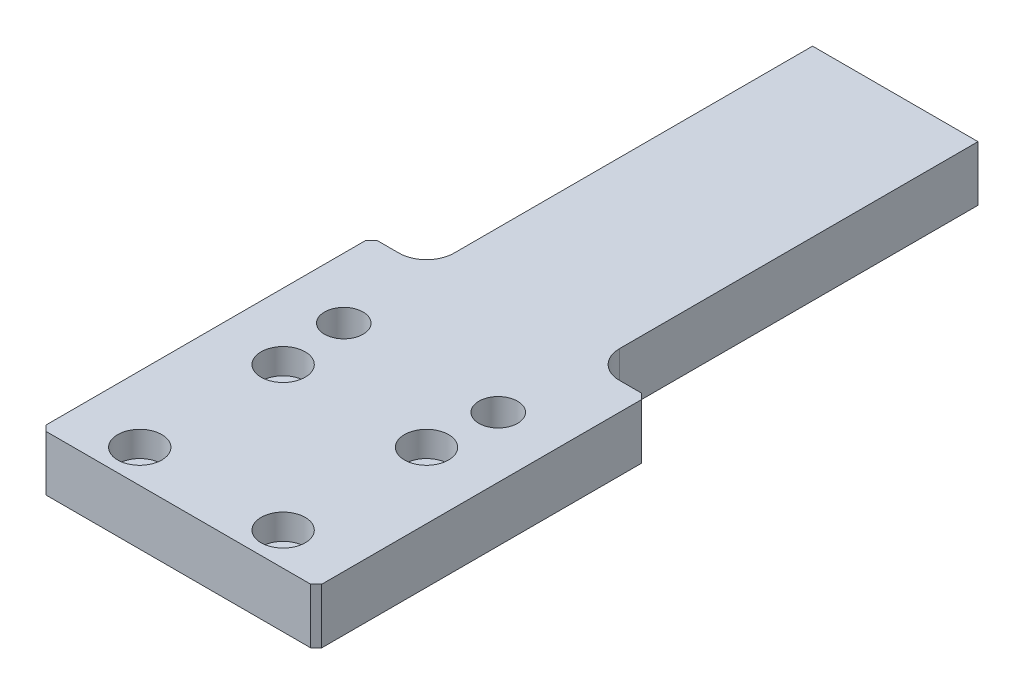
SolidWorks part; units mm, degrees
material "A6061"
ref_plane "前基準面" through (0, 0, 0) normal (0, 0, 1) x (1, 0, 0)
ref_plane "上基準面" through (0, 0, 0) normal (0, 1, 0) x (1, 0, 0)
ref_plane "右基準面" through (0, 0, 0) normal (1, 0, 0) x (0, 0, -1)
sketch "草图1" plane through (0, 0, 0) normal (0, 1, 0) x (1, 0, 0)
  line L1 (-25, -30) -> (25, -30)
  line L2 (-25, -30) -> (-25, 30)
  line L3 (-25, 30) -> (25, 30)
  line L4 (25, -30) -> (25, 30)
  line L5 (-25, -30) -> (25, 30) construction
  line L6 (-25, 30) -> (25, -30) construction
  point P0 (0, 0)
  dimension "D1" = 50
  dimension "D2" = 60
extrude "凸台-拉伸1" add sketch "草图1" along normal mid plane 10
hole_wizard "打孔尺寸(%根据)内六角圆柱头螺钉的类型1" positions "草图2" profile "草图3" counterbore size "M4" standard "GB" end condition through all
sketch "草图2" plane through (0, 5, 0) normal (0, 1, 0) x (1, 0, 0)
  line L0 (0, -40.7311) -> (0, 0) construction
  line L2 (-25, -30) -> (25, -30) construction
  point P0 (13, -24)
  point P2 (13, 2)
  point P10 (-13, 2)
  point P11 (-13, -24)
  dimension "D1" = 26
  dimension "D2" = 26
  dimension "D3" = 6
sketch "草图3" plane through (13, 5, 24) normal (1, 0, 0) x (0, 0, 1)
  line L0 (0, 0) -> (0, 10)
  line L1 (0, 10) -> (2.25, 10)
  line L3 (2.25, 10) -> (2.25, 4.6)
  line L4 (2.25, 4.6) -> (4, 4.6)
  line L5 (4, 4.6) -> (4, 0)
  line L7 (4, 0) -> (0, 0)
  line L11 (0, -6.35) -> (0, 107.95) construction
  dimension "通孔孔直径" = 4.5
  dimension "通孔孔深度" = 10
  dimension "柱形沉头孔直径" = 8
  dimension "柱形沉头孔深度" = 4.6
hole_wizard "M8x1.0 螺纹孔1" positions "草图6" profile "草图7" tap size "M8x1.0" standard "GB" end condition through all
sketch "草图6" plane through (0, 5, 0) normal (0, 1, 0) x (1, 0, 0)
  line L0 (0, 0) -> (0, 23.5494) construction
  line L2 (25, 30) -> (-25, 30) construction
  point P0 (-14, 14)
  point P2 (14, 14)
  dimension "D1" = 28
  dimension "D2" = 16
sketch "草图7" plane through (-14, 5, -14) normal (1, 0, 0) x (0, 0, 1)
  line L0 (0, 0) -> (0, 10)
  line L1 (0, 10) -> (3.5, 10)
  line L2 (3.5, 10) -> (3.5, 0)
  line L5 (3.5, 0) -> (0, 0)
  line L11 (0, -6.35) -> (0, 107.95) construction
  dimension "通孔螺纹孔钻头直径" = 7
  dimension "通孔螺纹孔钻头深度" = 10
cosmetic thread "孔螺蚊线4" parameters "D2"=8
cosmetic thread "孔螺蚊线5" parameters "D2"=8
sketch "草图8" plane through (0, 5, 0) normal (0, 1, 0) x (1, 0, 0)
  line L0 (25, 30) -> (-25, 30) construction
  line L1 (15, 30) -> (-15, 30)
  line L2 (15, 30) -> (15, 100)
  line L3 (15, 100) -> (-15, 100)
  line L4 (-15, 30) -> (-15, 100)
  line L5 (0, 0) -> (0, 30) construction
  dimension "D1" = 30
  dimension "D2" = 70
extrude "凸台-拉伸2" add sketch "草图8" against normal up to surface (10 mm away) up to face at (-14, -5, -10.5)
chamfer "倒角1" distance 1 angle 45 4 edges at (25, 0, -30) (-25, 0, -30) (25, 0, 30) (-25, 0, 30)
fillet "圆角1" radius 5 2 edges at (-15, 0, -30) (15, 0, -30)
hole_wizard "M4 螺纹孔1" positions "草图9" profile "草图10" tap size "M4" standard "GB"
sketch "草图9" plane through (0, 0, -100) normal (0, 0, -1) x (-1, 0, 0)
  line L0 (0, -8.9893) -> (0, 0) construction
  point P0 (10, 0)
  point P8 (-10, 0)
  dimension "D1" = 20
sketch "草图10" plane through (-10, 0, -100) normal (1, 0, 0) x (0, 1, 0)
  line L0 (0, 0) -> (0, 11.0914)
  line L1 (0, 11.0914) -> (1.65, 10.1)
  line L2 (1.65, 10.1) -> (1.65, 0)
  line L5 (1.65, 0) -> (0, 0)
  line L10 (0, 11.0914) -> (-1.65, 10.1) construction
  line L11 (0, -6.35) -> (0, 107.95) construction
  dimension "螺纹孔钻头直径" = 3.3
  dimension "螺纹孔钻头深度" = 10.1
  dimension "导头角度" = 118
cosmetic thread "孔螺蚊线6" parameters "D1"=8, "D2"=4
cosmetic thread "孔螺蚊线7" parameters "D1"=8, "D2"=4
